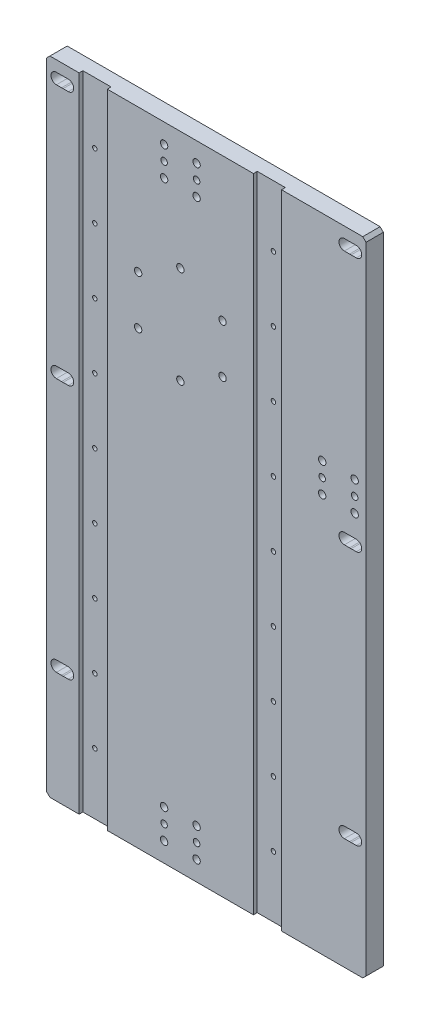
from build123d import *

# Parameters (mm, degrees)
SKETCH1_W                    = 295
SKETCH1_H                    = 593
EXTRUDE1_DEPTH               = 8
CUT_EXTRUDE1_DEPTH           = 3.5
CHAMFER1_SIZE                = 3
CUT_EXTRUDE2_DEPTH           = 30
M8_TAPPED_HOLE1_D            = 6.8
M8_TAPPED_HOLE1_DEPTH        = 22.25
M8_TAPPED_HOLE1_TIP          = 2.042926105
SKETCH6_R                    = 5.05
CUT_EXTRUDE3_DEPTH           = 20
M8_TAPPED_HOLE2_D            = 6.8
SIZE_MM_BLIND_DOWEL_HOLE_1_D = 6
M8_TAPPED_HOLE3_D            = 6.8
SIZE_MM_BLIND_DOWEL_HOLE_2_D = 6
M5_TAPPED_HOLE1_D            = 4.2


with BuildPart() as part:
    # Sketch1 → Extrude1 (new, symmetric)
    with BuildSketch(Plane.XY):
        Rectangle(SKETCH1_W, SKETCH1_H)
    extrude(amount=EXTRUDE1_DEPTH, both=True)

    # 草图1 → Cut-Extrude1 (cut)
    with BuildSketch(Plane.XY.offset(8)):
        with BuildLine():
            Line((-91.5, 333.5), (-91.5, -316.5))
            ThreePointArc((-91.5, -316.5), (-104.5, -329.5), (-117.5, -316.5))
            Line((-117.5, -316.5), (-117.5, 333.5))
            ThreePointArc((-117.5, 333.5), (-104.5, 346.5), (-91.5, 333.5))
        make_face()
        with BuildLine():
            Line((69.5, 333.5), (69.5, -316.5))
            ThreePointArc((69.5, -316.5), (56.5, -329.5), (43.5, -316.5))
            Line((43.5, -316.5), (43.5, 333.5))
            ThreePointArc((43.5, 333.5), (56.5, 346.5), (69.5, 333.5))
        make_face()
    extrude(amount=-CUT_EXTRUDE1_DEPTH, mode=Mode.SUBTRACT)

    # Chamfer1
    chamfer1_edges = [part.edges().sort_by_distance(p)[0] for p in [
        (-147.5, 296.5, 0),
        (147.5, 296.5, 0),
        (147.5, -296.5, 0),
        (-147.5, -296.5, 0),
    ]]
    chamfer(chamfer1_edges, length=CHAMFER1_SIZE)

    # Sketch2 → Cut-Extrude2 (cut)
    with BuildSketch(Plane.XY.offset(8)):
        with BuildLine():
            Line((138.5, 276.5), (127.5, 276.5))
            ThreePointArc((127.5, 276.5), (122.5, 281.5), (127.5, 286.5))
            Line((127.5, 286.5), (138.5, 286.5))
            ThreePointArc((138.5, 286.5), (143.5, 281.5), (138.5, 276.5))
        make_face()
        with BuildLine():
            Line((-127.5, 276.5), (-138.5, 276.5))
            ThreePointArc((-138.5, 276.5), (-143.5, 281.5), (-138.5, 286.5))
            Line((-138.5, 286.5), (-127.5, 286.5))
            ThreePointArc((-127.5, 286.5), (-122.5, 281.5), (-127.5, 276.5))
        make_face()
        with BuildLine():
            Line((-127.5, -193.5), (-138.5, -193.5))
            ThreePointArc((-138.5, -193.5), (-143.5, -188.5), (-138.5, -183.5))
            Line((-138.5, -183.5), (-127.5, -183.5))
            ThreePointArc((-127.5, -183.5), (-122.5, -188.5), (-127.5, -193.5))
        make_face()
        with BuildLine():
            Line((-127.5, 41.5), (-138.5, 41.5))
            ThreePointArc((-138.5, 41.5), (-143.5, 46.5), (-138.5, 51.5))
            Line((-138.5, 51.5), (-127.5, 51.5))
            ThreePointArc((-127.5, 51.5), (-122.5, 46.5), (-127.5, 41.5))
        make_face()
        with BuildLine():
            Line((138.5, -193.5), (127.5, -193.5))
            ThreePointArc((127.5, -193.5), (122.5, -188.5), (127.5, -183.5))
            Line((127.5, -183.5), (138.5, -183.5))
            ThreePointArc((138.5, -183.5), (143.5, -188.5), (138.5, -193.5))
        make_face()
        with BuildLine():
            Line((138.5, 41.5), (127.5, 41.5))
            ThreePointArc((127.5, 41.5), (122.5, 46.5), (127.5, 51.5))
            Line((127.5, 51.5), (138.5, 51.5))
            ThreePointArc((138.5, 51.5), (143.5, 46.5), (138.5, 41.5))
        make_face()
    extrude(amount=-CUT_EXTRUDE2_DEPTH, mode=Mode.SUBTRACT)

    # M8 Tapped Hole1
    with Locations(Plane.XY.offset(8)):
        with Locations((14.97114317, 164.5), (14.97114317, 119.5), (-24, 97), (-62.97114317, 119.5), (-62.97114317, 164.5), (-24, 187)):
            Hole(M8_TAPPED_HOLE1_D / 2, depth=M8_TAPPED_HOLE1_DEPTH)
            with Locations((0, 0, -(M8_TAPPED_HOLE1_DEPTH + M8_TAPPED_HOLE1_TIP / 2))):  # 118° drill point
                Cone(0, M8_TAPPED_HOLE1_D / 2, M8_TAPPED_HOLE1_TIP, mode=Mode.SUBTRACT)

    # Sketch6 → Cut-Extrude3 (cut)
    with BuildSketch(Plane.XY.offset(8)):
        with Locations((-133, 281.5)):
            Circle(SKETCH6_R)
        with Locations((133, 281.5)):
            Circle(SKETCH6_R)
        with Locations((-133, 46.5)):
            Circle(SKETCH6_R)
        with Locations((133, 46.5)):
            Circle(SKETCH6_R)
        with Locations((-133, -188.5)):
            Circle(SKETCH6_R)
        with Locations((133, -188.5)):
            Circle(SKETCH6_R)
    extrude(amount=-CUT_EXTRUDE3_DEPTH, mode=Mode.SUBTRACT)

    # M8 Tapped Hole2 (through all)
    with Locations(Plane.XY.offset(8)):
        with Locations((107, 71.5), (137, 71.5), (137, 98.5), (107, 98.5)):
            Hole(M8_TAPPED_HOLE2_D / 2)

    # Size mm blind dowel hole 1 (through all)
    with Locations(Plane.XY.offset(8)):
        with Locations((107, 85), (137, 85)):
            Hole(SIZE_MM_BLIND_DOWEL_HOLE_1_D / 2)

    # M8 Tapped Hole3 (through all)
    with Locations(Plane.XY.offset(8)):
        with Locations((-9, 278.5), (-9, 251.5), (-39, 278.5), (-39, 251.5), (-9, -251.5), (-9, -278.5), (-39, -278.5), (-39, -251.5)):
            Hole(M8_TAPPED_HOLE3_D / 2)

    # Size mm blind dowel hole 2 (through all)
    with Locations(Plane.XY.offset(8)):
        with Locations((-9, 265), (-39, 265), (-9, -265), (-39, -265)):
            Hole(SIZE_MM_BLIND_DOWEL_HOLE_2_D / 2)

    # M5 Tapped Hole1 (through all)
    with Locations(Plane.XY.offset(4.5)):
        with Locations((58.5, 240), (58.5, 180), (58.5, 120), (58.5, 60), (58.5, 0), (58.5, -60), (58.5, -120), (58.5, -180), (58.5, -240), (-106.5, -240), (-106.5, -180), (-106.5, -120), (-106.5, -60), (-106.5, 0), (-106.5, 60), (-106.5, 120), (-106.5, 180), (-106.5, 240)):
            Hole(M5_TAPPED_HOLE1_D / 2)


solid = part.part
